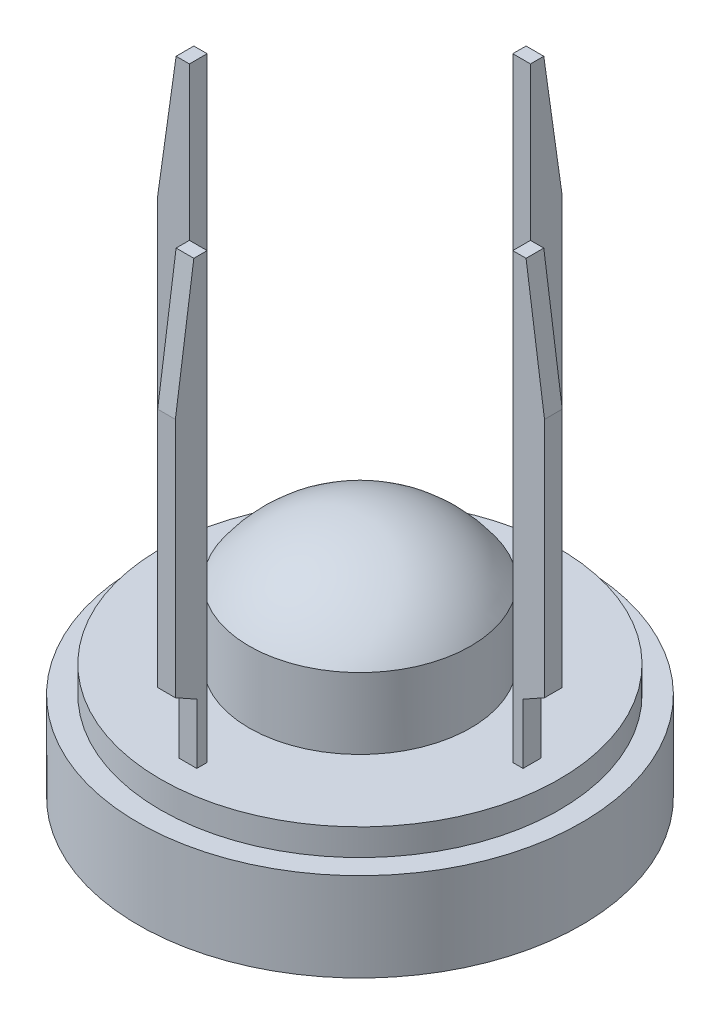
from build123d import *

# Parameters (mm, degrees)
SKETCH1_W           = 250
SKETCH1_H           = 100
SKETCH2_R           = 225
BOSS_EXTRUDE1_DEPTH = 30
SKETCH3_R           = 125
BOSS_EXTRUDE2_DEPTH = 80
BOSS_EXTRUDE3_DEPTH = 10
CIRPATTERN1_COUNT   = 4


with BuildPart() as part:
    # Sketch1 → Revolve1 (revolve)
    with BuildSketch(Plane.XY, mode=Mode.PRIVATE) as revolve1_sk:
        with Locations((125, 50)):
            Rectangle(SKETCH1_W, SKETCH1_H)
    revolve(revolve1_sk.sketch.rotate(Axis((0, 0, 0), (0, 1, 0)), 90), axis=Axis((0, 0, 0), (0, 1, 0)))

    # Sketch2 → Boss-Extrude1 (add)
    with BuildSketch(Plane(origin=(0, 100, 0), x_dir=(1, 0, 0), z_dir=(0, 1, 0))):
        with Locations(Location((0, 0, 0), (0, 0, 270))):
            Circle(SKETCH2_R)
    extrude(amount=BOSS_EXTRUDE1_DEPTH)

    # Sketch3 → Boss-Extrude2 (add)
    with BuildSketch(Plane(origin=(0, 130, 0), x_dir=(1, 0, 0), z_dir=(0, 1, 0))):
        with Locations(Location((0, 0, 0), (0, 0, 270))):
            Circle(SKETCH3_R)
    extrude(amount=BOSS_EXTRUDE2_DEPTH)

    # Sketch4 → Revolve2 (revolve)
    with BuildSketch(Plane.XY):
        with BuildLine():
            Line((0, 210), (0, 275.518788168))
            ThreePointArc((0, 275.518788168), (70.565061473, 258.146319153), (125, 210))
            Line((125, 210), (0, 210))
        make_face()
    revolve(axis=Axis((0, 210, 0), (0, 1, 0)))

    # Sketch5 → Boss-Extrude3 (add, symmetric)
    with BuildSketch(Plane.XY):
        Polygon((-194.003425054, 130), (-182.358299763, 130), (-182.358299763, 145.262915146), (-182.358299763, 630), (-197.365341888, 630), (-218.16183032, 483.058469024), (-218.16183032, 211.101864805), (-194.003425054, 197.687306821), align=None)
    boss_extrude3 = extrude(amount=BOSS_EXTRUDE3_DEPTH, both=True)

    # CirPattern1: Boss-Extrude3 ×4 about axis
    cirpattern1_axis = Axis((0, 0, 0), (0, 1, 0))
    for i in range(1, CIRPATTERN1_COUNT):
        add(boss_extrude3.rotate(cirpattern1_axis, i * 360 / CIRPATTERN1_COUNT))


solid = part.part
